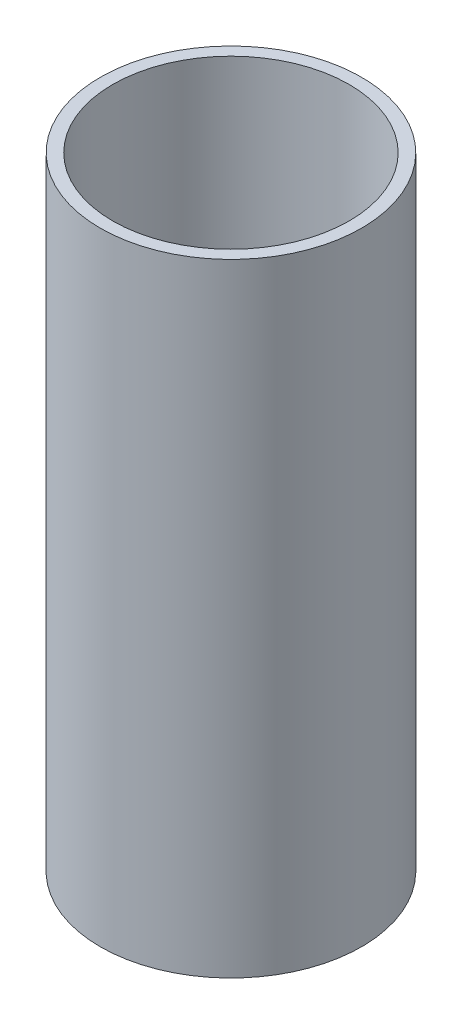
from build123d import *

# Parameters (mm, degrees)
SKETCH1_R           = 10.5
SKETCH1_R_2         = 9.5
BOSS_EXTRUDE1_DEPTH = 50


with BuildPart() as part:
    # Sketch1 → Boss-Extrude1 (new body)
    with BuildSketch(Plane(origin=(0, 0, 0), x_dir=(1, 0, 0), z_dir=(0, 1, 0))):
        with Locations(Location((0, 0, 0), (0, 0, 270))):
            Circle(SKETCH1_R)
        with Locations(Location((0, 0, 0), (0, 0, 270))):
            Circle(SKETCH1_R_2, mode=Mode.SUBTRACT)
    extrude(amount=BOSS_EXTRUDE1_DEPTH)


solid = part.part
